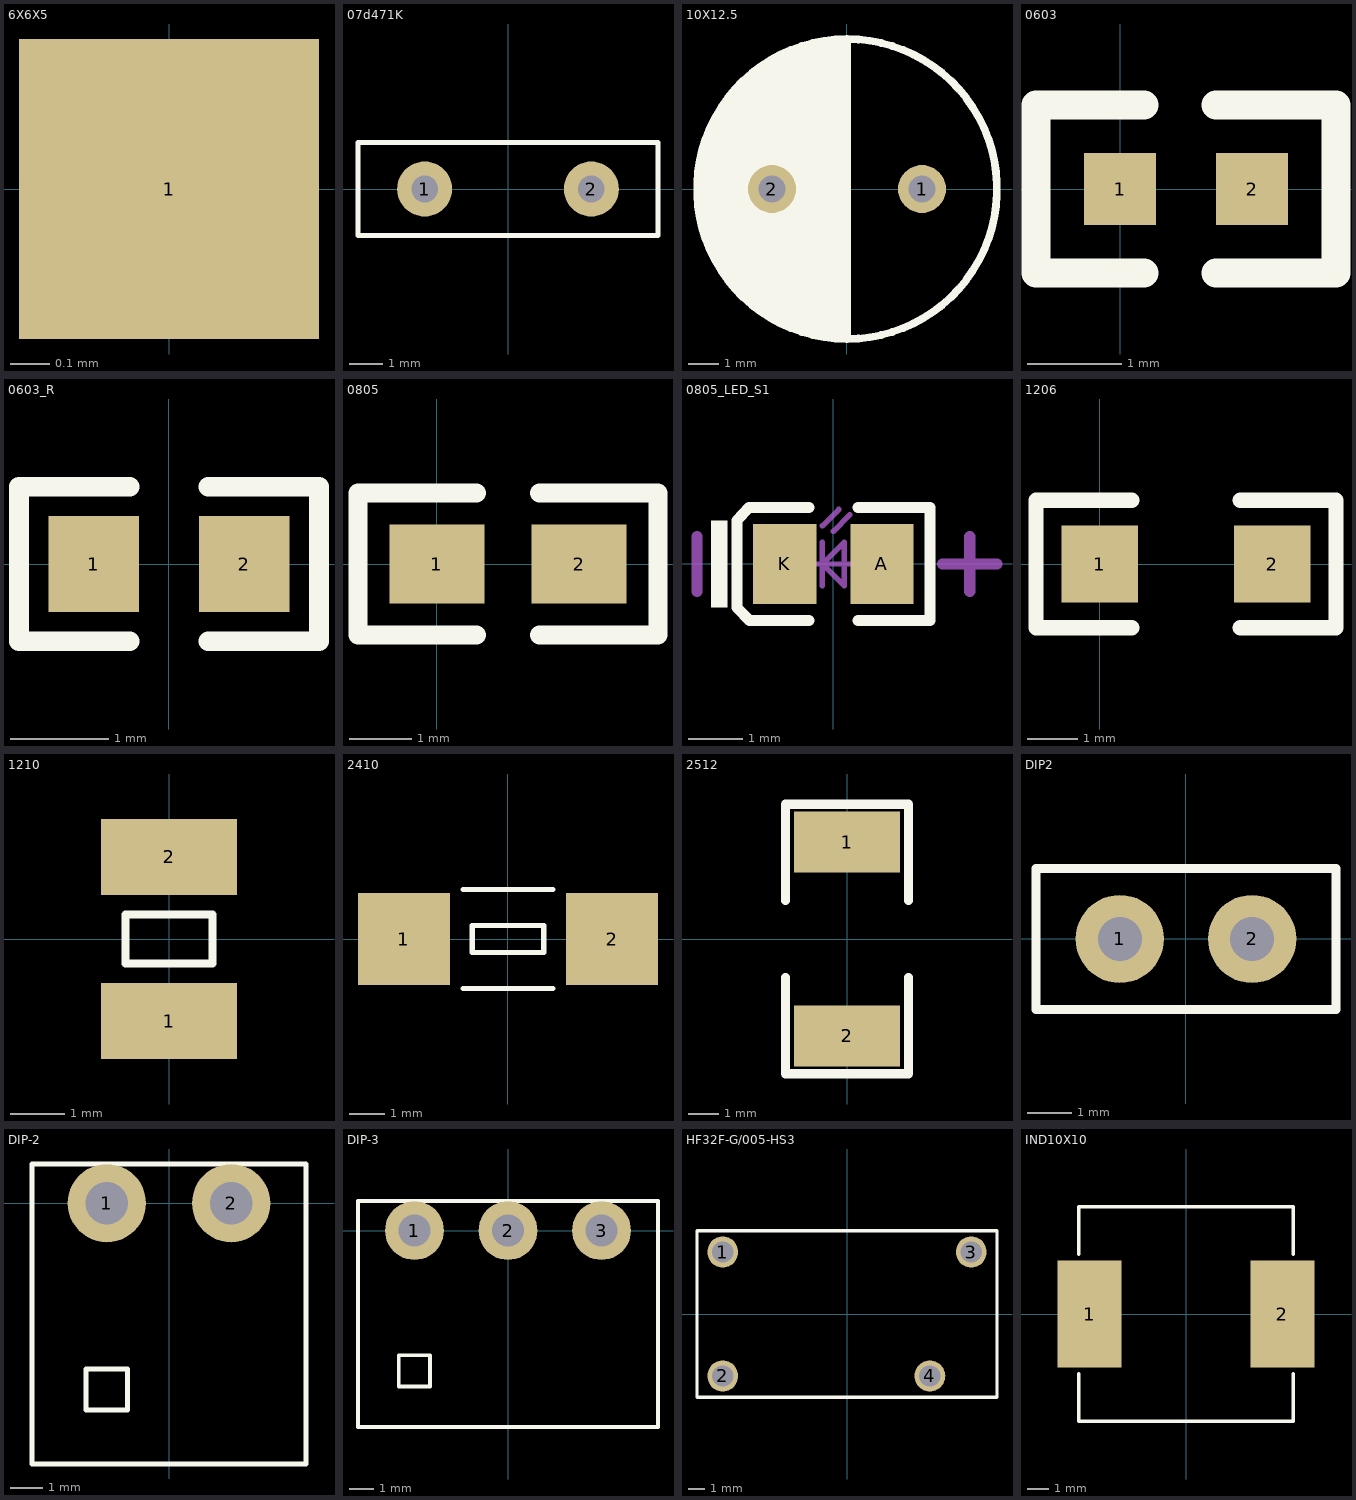
[diagram p0: the footprints below, top view; thin cyan lines are the x and y axes]
# Altium footprint library MISC82282.PcbLib: 24 footprints (part 1 of 2)
Each footprint in its own frame and in the unit in brackets; x right, y up, seen from the top. Pads: shape width x height; smd on the part's side, far side on the other; paste and mask are expansions set on the pad; w line width, h text height; cw(c..) or ccw(c..) is an arc to the next point about the centre after c.

## 6X6X5 [mil]
pads (1):
  rect 30x30 smd: 1(0,0)

## 07d471K [mm]
pads (2):
  round 1.65 hole 0.8: 1(-2.5,0) 2(2.5,0)
Top Overlay:
  lines w0.15: -4.5,-1.4 -4.5,1.4 4.5,1.4 4.5,-1.4 -4.5,-1.4

## 10X12.5 [mm]
pads (2):
  round 1.6 hole 0.9: 1(2.5,0) 2(-2.5,0)
Top Overlay:
  region: 0,-5 -0.328,-5 -0.978,-4.914 -1.611,-4.745 -2.216,-4.494 -2.784,-4.166 -3.304,-3.767 -3.767,-3.304 -4.166,-2.784 -4.494,-2.216 -4.745,-1.611 -4.914,-0.978 -5,-0.328 -5,0.328 -4.914,0.978 -4.745,1.611 -4.494,2.216 -4.166,2.784 -3.767,3.304 -3.304,3.767 -2.784,4.166 -2.216,4.494 -1.611,4.745 -0.978,4.914 -0.328,5 0,5
  lines w0.254: 0,-4.978 0,0 0,4.978 ; 0,-5 cw(c0,0) 0,5 cw(c0,0) 0,-5
3D body: height 14, standoff -3.5, extent -5.002,-4.993 5,4.993

## 0603 [mil]
height 156.69
pads (2):
  rect 30x30 smd: 1(0,0) 2(55,0)
Top Overlay:
  lines w12: 10,-35 -35,-35 -35,35 10,35 ; 40,-35 90,-35 90,35 40,35

## 0603_R [mm]
height 3.98
pads (2):
  rect 0.93x0.98 smd: 1(-0.77,0) 2(0.77,0)
Top Overlay:
  lines w0.2: -0.4,-0.79 -1.535,-0.79 -1.535,0.79 -0.4,0.79 ; 0.4,-0.79 1.535,-0.79 1.535,0.79 0.4,0.79
3D body: height 0.56, standoff 0, extent -0.85,-0.4 0.85,0.4

## 0805 [mil]
pads (2):
  rect 60x50 smd: 1(0,0) 2(90,0)
Top Overlay:
  lines w12: 25,-45 -50,-45 -50,45 25,45 ; 65,-45 140,-45 140,45 65,45

## 0805_LED_S1 [mm]
height 3.98
pads (2):
  rect 1.16x1.47 smd: A(0.89,0) K(-0.89,0)
Top Overlay:
  rectangle: -2.245,-0.8 -1.945,0.8
  lines w0.2: -0.45,-1.035 -1.535,-1.035 -1.77,-0.8 -1.77,0.8 -1.55,1.035 -0.45,1.035 ; 0.45,-1.035 1.77,-1.035 1.77,1.035 0.45,1.035
Mechanical 13:
  lines w0.1: -0.4,0 0.4,0 ; -0.2,-0.4 -0.2,0.4 ; -0.2,0.7 0.1,1 ; 0,0.6 0.3,0.9 ; -0.2,0 0.2,0.4 0.2,-0.4 -0.2,0
Mechanical 15:
  lines w0.203: -2.5,-0.5 -2.5,0.5 ; 2,0 3,0 ; 2.5,-0.5 2.5,0.5
3D body: height 1.1, standoff 0, extent -1.01,-0.625 1.01,0.625

## 1206 [mil]
pads (2):
  rect 60x60 smd: 1(0,0) 2(135,0)
Top Overlay:
  lines w12: 25,-50 -50,-50 -50,50 25,50 ; 110,-50 185,-50 185,50 110,50

## 1210 [mm]
pads (2):
  rect 2.5x1.4 smd: 1(0,-1.515) 2(0,1.515)
Top Overlay:
  lines w0.152: -0.8,-0.45 -0.8,0.45 0.8,0.45 0.8,-0.45 -0.8,-0.45

## 2410 [mm]
pads (2):
  rect 2.6x2.6 smd: 1(-2.95,0) 2(2.95,0)
Top Overlay:
  lines w0.15: -1.27,-1.4 1.27,-1.4 ; -1.27,1.4 1.27,1.4 ; -1.016,-0.381 1.016,-0.381 1.016,0.381 -1.016,0.381 -1.016,-0.381

## 2512 [mm]
pads (2):
  rect 3.5x2 smd: 1(0,3.2) 2(0,-3.2)
Top Overlay:
  lines w0.305: -2.032,-1.27 -2.032,-4.445 2.032,-4.445 2.032,-1.27 ; -2.032,1.27 -2.032,4.445 2.032,4.445 2.032,1.27
3D body: height 0.6, standoff 0, extent -1.6,-3.2 1.6,3.2

## DIP2 [mm]
height 3.98
pads (2):
  round 2 hole 1: 1(-1.5,0) 2(1.5,0)
Top Overlay:
  lines w0.2: 3.331,-1.6 -3.4,-1.6 -3.4,1.6 3.4,1.6 3.4,-1.6

## DIP-2 [mm]
pads (2):
  round 2.4 hole 1.3: 1(-1.905,0) 2(1.905,0)
Top Overlay:
  lines w0.152: -4.205,-8 -4.205,1.2 4.205,1.2 4.205,-8 -4.205,-8 ; -2.54,-6.35 -2.54,-5.08 -1.27,-5.08 -1.27,-6.35 -2.54,-6.35

## DIP-3 [mm]
pads (3):
  round 2.4 hole 1.3: 1(-3.81,0) 2(0,0) 3(3.81,0)
Top Overlay:
  lines w0.152: -6.11,-8 -6.11,1.2 6.11,1.2 6.11,-8 -6.11,-8 ; -4.445,-6.35 -4.445,-5.08 -3.175,-5.08 -3.175,-6.35 -4.445,-6.35

## HF32F-G/005-HS3 [mm]
pads (4):
  round 1.9 hole 1.3: 1(-7.62,3.8) 2(-7.62,-3.8) 3(7.62,3.8) 4(5.08,-3.8)
Top Overlay:
  lines w0.2: -9.2,-5.1 -9.2,5.1 9.2,5.1 9.2,-5.1 -9.2,-5.1

## IND10X10 [mm]
pads (2):
  rect 3x5 smd: 1(-4.5,0) 2(4.5,0)
Top Overlay:
  lines w0.152: -5,-2.794 -5,-5 5,-5 5,-2.794 ; -5,2.794 -5,5 5,5 5,2.794